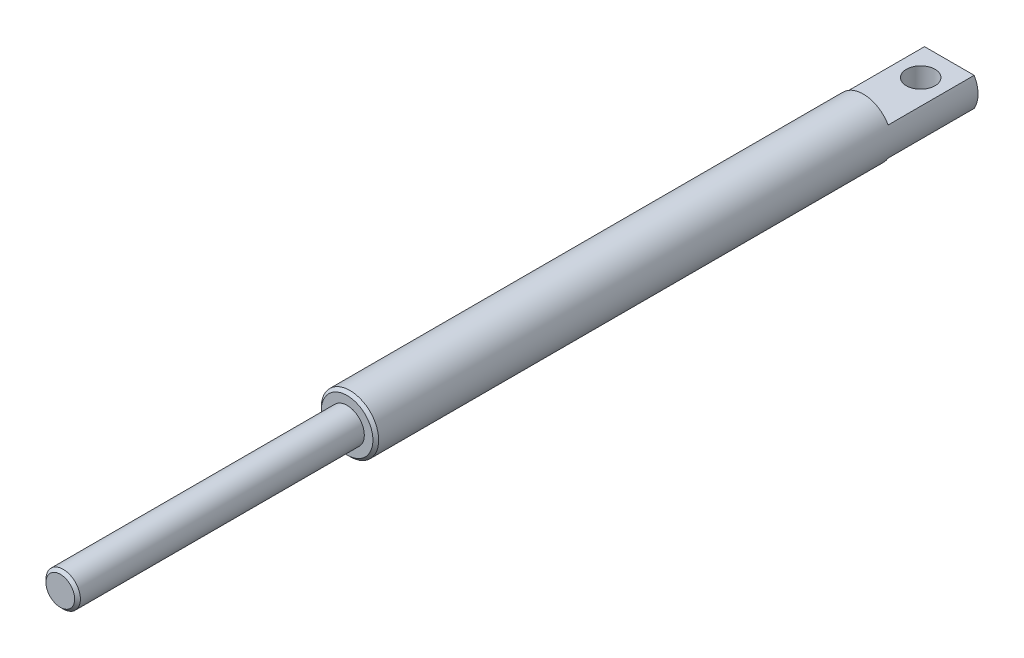
from build123d import *

# Parameters (mm, degrees)
SKETCH1_R               = 10
BOSS_EXTRUDE1_DEPTH     = 210
CUT_EXTRUDE1_DEPTH      = 211.475651798
CUT_EXTRUDE1_DEPTH_BACK = 211.475651798
SKETCH2_R               = 5
CUT_EXTRUDE2_DEPTH      = 211.475651908
CUT_EXTRUDE2_DEPTH_BACK = 30
SKETCH3_W               = 38.012097267
SKETCH3_H               = 10.508452135
SKETCH3_W_2             = 32.719606191
SKETCH3_H_2             = 9.885466079
SKETCH4_R               = 6
BOSS_EXTRUDE2_DEPTH     = 100
CHAMFER1_SIZE           = 1


with BuildPart() as part:
    # Sketch1 → Boss-Extrude1 (new body)
    with BuildSketch(Plane.XY):
        Circle(SKETCH1_R)
    extrude(amount=BOSS_EXTRUDE1_DEPTH)

    # Sketch2 → Cut-Extrude1 (cut, two sides: drawn at the far end of the back side and taken through both)
    with BuildSketch(Plane(origin=(0, 0, 0), x_dir=(1, 0, 0), z_dir=(0, 1, 0)).offset(-CUT_EXTRUDE1_DEPTH_BACK)):
        with Locations(Location((0, -10, 0), (0, 0, 270))):
            Circle(SKETCH2_R)
    extrude(amount=CUT_EXTRUDE1_DEPTH + CUT_EXTRUDE1_DEPTH_BACK, mode=Mode.SUBTRACT)

    # Sketch3 → Cut-Extrude2 (cut, two sides: drawn at the far end of the back side and taken through both)
    with BuildSketch(Plane(origin=(0, 0, 0), x_dir=(-1, 0, 0), z_dir=(0, 0, -1)).offset(-CUT_EXTRUDE2_DEPTH_BACK)):
        with Locations((0.51811282, -10.254226067)):
            Rectangle(SKETCH3_W, SKETCH3_H)
        with Locations((1.092602531, 9.94273304)):
            Rectangle(SKETCH3_W_2, SKETCH3_H_2)
    extrude(amount=CUT_EXTRUDE2_DEPTH + CUT_EXTRUDE2_DEPTH_BACK, mode=Mode.SUBTRACT)

    # Sketch4 → Boss-Extrude2 (add)
    with BuildSketch(Plane.XY.offset(210)):
        Circle(SKETCH4_R)
    extrude(amount=BOSS_EXTRUDE2_DEPTH)

    # Chamfer1
    chamfer1_edges = [part.edges().sort_by_distance(p)[0] for p in [
        (-10, 0, 210),
        (-6, 0, 310),
    ]]
    chamfer(chamfer1_edges, length=CHAMFER1_SIZE)


solid = part.part
